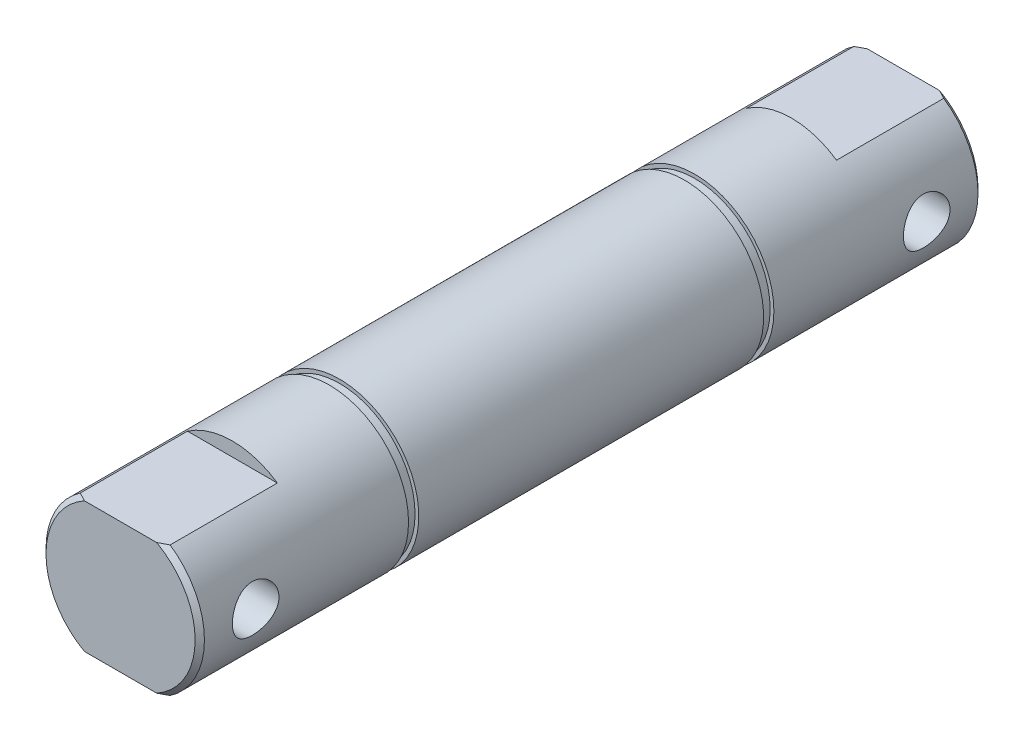
SolidWorks part; units mm, degrees
ref_plane "前视" through (0, 0, 0) normal (0, 0, 1) x (1, 0, 0)
ref_plane "上视" through (0, 0, 0) normal (0, 1, 0) x (1, 0, 0)
ref_plane "右视" through (0, 0, 0) normal (1, 0, 0) x (0, 0, -1)
sketch "草图1" plane through (0, 0, 0) normal (0, 0, 1) x (1, 0, 0)
  circle A0 centre (0, 0) radius 8.5
  dimension "D1" = 17
extrude "凸台-拉伸1" add sketch "草图1" along normal mid plane 84
sketch "草图2" plane through (0, 0, 42) normal (0, 0, 1) x (1, 0, 0)
  line L0 (0, 8.5) -> (0, -8.5) construction
  line L1 (-12.5, 10) -> (12.5, 10)
  line L2 (-12.5, 10) -> (-12.5, 7)
  line L3 (-12.5, 7) -> (12.5, 7)
  line L4 (12.5, 10) -> (12.5, 7)
  line L5 (-12.5, 10) -> (12.5, 7) construction
  line L6 (-12.5, 7) -> (12.5, 10) construction
  line L7 (0, 0) -> (8.5, 0) construction
  line L8 (-12.5, -7) -> (12.5, -10) construction
  line L9 (-12.5, -10) -> (12.5, -7) construction
  line L10 (12.5, -10) -> (12.5, -7)
  line L11 (-12.5, -7) -> (12.5, -7)
  line L12 (-12.5, -10) -> (-12.5, -7)
  line L13 (-12.5, -10) -> (12.5, -10)
  circle A0 centre (0, 0) radius 8.5 construction
  point P0 (0, 8.5)
  dimension "D1" = 25
  dimension "D2" = 14
extrude "切除-拉伸1" cut sketch "草图2" against normal blind 12
mirror "镜向1" about plane through (0, 0, 0) normal (0, 0, 1) of "切除-拉伸1"
chamfer "倒角2" distance 0.5 angle 45 4 edges at (8.5, 0, -42) (-8.5, 0, -42) (8.5, 0, 42) (-8.5, 0, 42)
ref_plane "基准面1" through (8.5, 0, 0) normal (1, 0, 0) x (0, 0, -1)
hole_wizard "M6 螺纹孔1" positions "草图4" profile "草图3" tap size "M6" standard "GB" end condition through all
sketch "草图4" plane through (8.5, 0, 0) normal (1, 0, 0) x (0, 0, -1)
  line L0 (-36, 0) -> (-42, 0) construction
  line L1 (-42, 7) -> (-42, -7) construction
  line L4 (36, 0) -> (42, 0) construction
  line L5 (42, -7) -> (42, 7) construction
  point P0 (-36, 0)
  point P2 (36, 0)
  dimension "D1" = 6
sketch "草图3" plane through (8.5, 0, 36) normal (0, 1, 0) x (0, 0, -1)
  line L0 (0, 0) -> (0, 17)
  line L1 (0, 17) -> (2.5, 17)
  line L2 (2.5, 17) -> (2.5, 0)
  line L5 (2.5, 0) -> (0, 0)
  line L11 (0, -6.35) -> (0, 107.95) construction
  dimension "通孔螺纹孔钻头直径" = 5
  dimension "通孔螺纹孔钻头深度" = 17
cosmetic thread "孔螺蚊线1" parameters "D2"=6
cosmetic thread "孔螺蚊线2" parameters "D2"=6
sketch "草图5" plane through (0, 0, 0) normal (0, 1, 0) x (1, 0, 0)
  line L0 (-8.5, 33.5) -> (-8.5, -33.5) construction
  line L1 (-8.5, 19.6) -> (-8.1, 19.6)
  line L2 (-8.5, 19.6) -> (-8.5, 18.5)
  line L3 (-8.5, 18.5) -> (-8.1, 18.5)
  line L4 (-8.1, 19.6) -> (-8.1, 18.5)
  line L5 (0, 0) -> (-23.4947, 0) construction
  line L6 (-8.5, -18.5) -> (-8.1, -18.5)
  line L7 (-8.5, -18.5) -> (-8.5, -19.6)
  line L8 (-8.5, -19.6) -> (-8.1, -19.6)
  line L9 (-8.1, -18.5) -> (-8.1, -19.6)
  line L10 (0, 0) -> (0, 18.5) construction
  dimension "D1" = 1.1
  dimension "D2" = 8.1
  dimension "D3" = 37
revolve "切除-旋转1" cut sketch "草图5" angle 360 about L10
